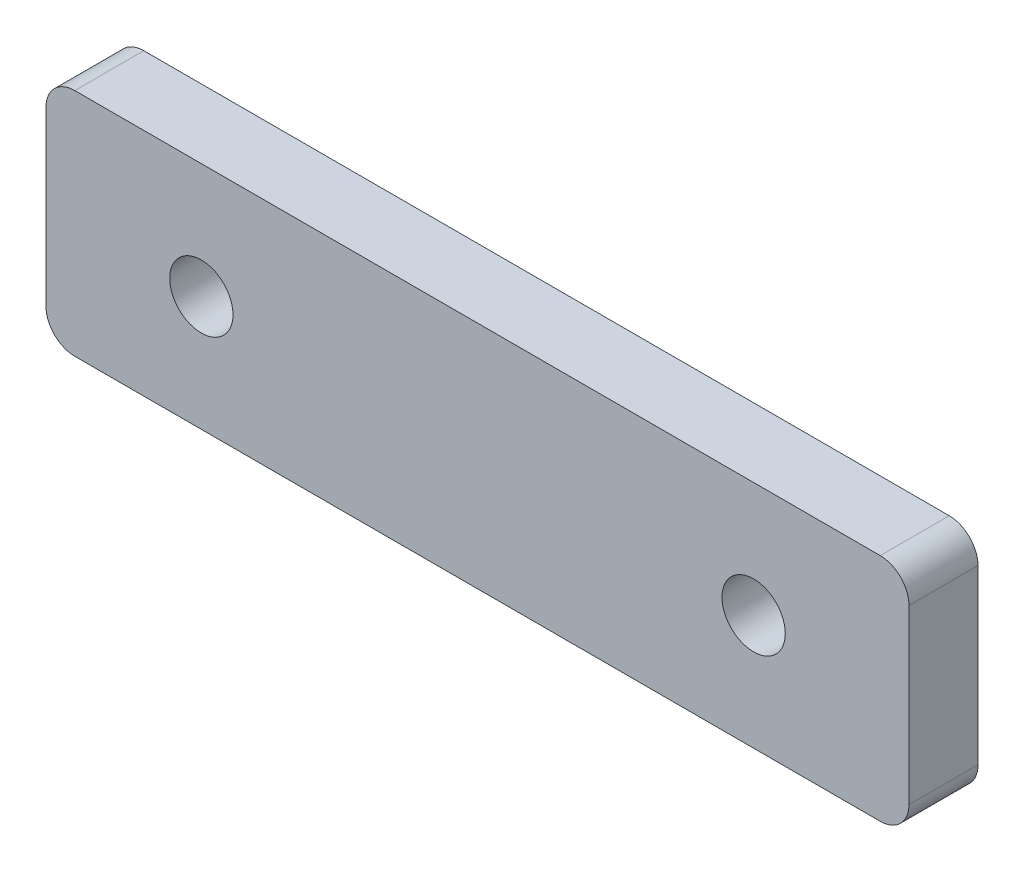
from build123d import *

# Parameters (mm, degrees)
SKETCH1_W           = 150
SKETCH1_H           = 40
BOSS_EXTRUDE1_DEPTH = 12
SKETCH2_R           = 5.5
CUT_EXTRUDE1_DEPTH  = 8
FILLET1_R           = 5
CUT_EXTRUDE2_START  = -12
SKETCH3_R           = 5.5
CUT_EXTRUDE2_DEPTH  = 12


with BuildPart() as part:
    # Sketch1 → Boss-Extrude1 (new body)
    with BuildSketch(Plane.XY):
        Rectangle(SKETCH1_W, SKETCH1_H)
    extrude(amount=BOSS_EXTRUDE1_DEPTH)

    # Sketch2 → Cut-Extrude1 (cut)
    with BuildSketch(Plane.XY.offset(12)):
        with Locations((-48, 0)):
            Circle(SKETCH2_R)
        with Locations((48, 0)):
            Circle(SKETCH2_R)
    extrude(amount=-CUT_EXTRUDE1_DEPTH, mode=Mode.SUBTRACT)

    # Fillet1
    fillet1_edges = [part.edges().sort_by_distance(p)[0] for p in [
        (75, -20, 6),
        (-75, -20, 6),
        (-75, 20, 6),
        (75, 20, 6),
    ]]
    fillet(fillet1_edges, radius=FILLET1_R)

    # Sketch3 → Cut-Extrude2 (cut)
    with BuildSketch(Plane(origin=(0, 0, 0), x_dir=(-1, 0, 0), z_dir=(0, 0, -1)).offset(CUT_EXTRUDE2_START)):
        with Locations(Location((-48, 0, 0), (0, 0, 180))):
            Circle(SKETCH3_R)
        with Locations(Location((48, 0, 0), (0, 0, 180))):
            Circle(SKETCH3_R)
    extrude(amount=CUT_EXTRUDE2_DEPTH, mode=Mode.SUBTRACT)


solid = part.part
